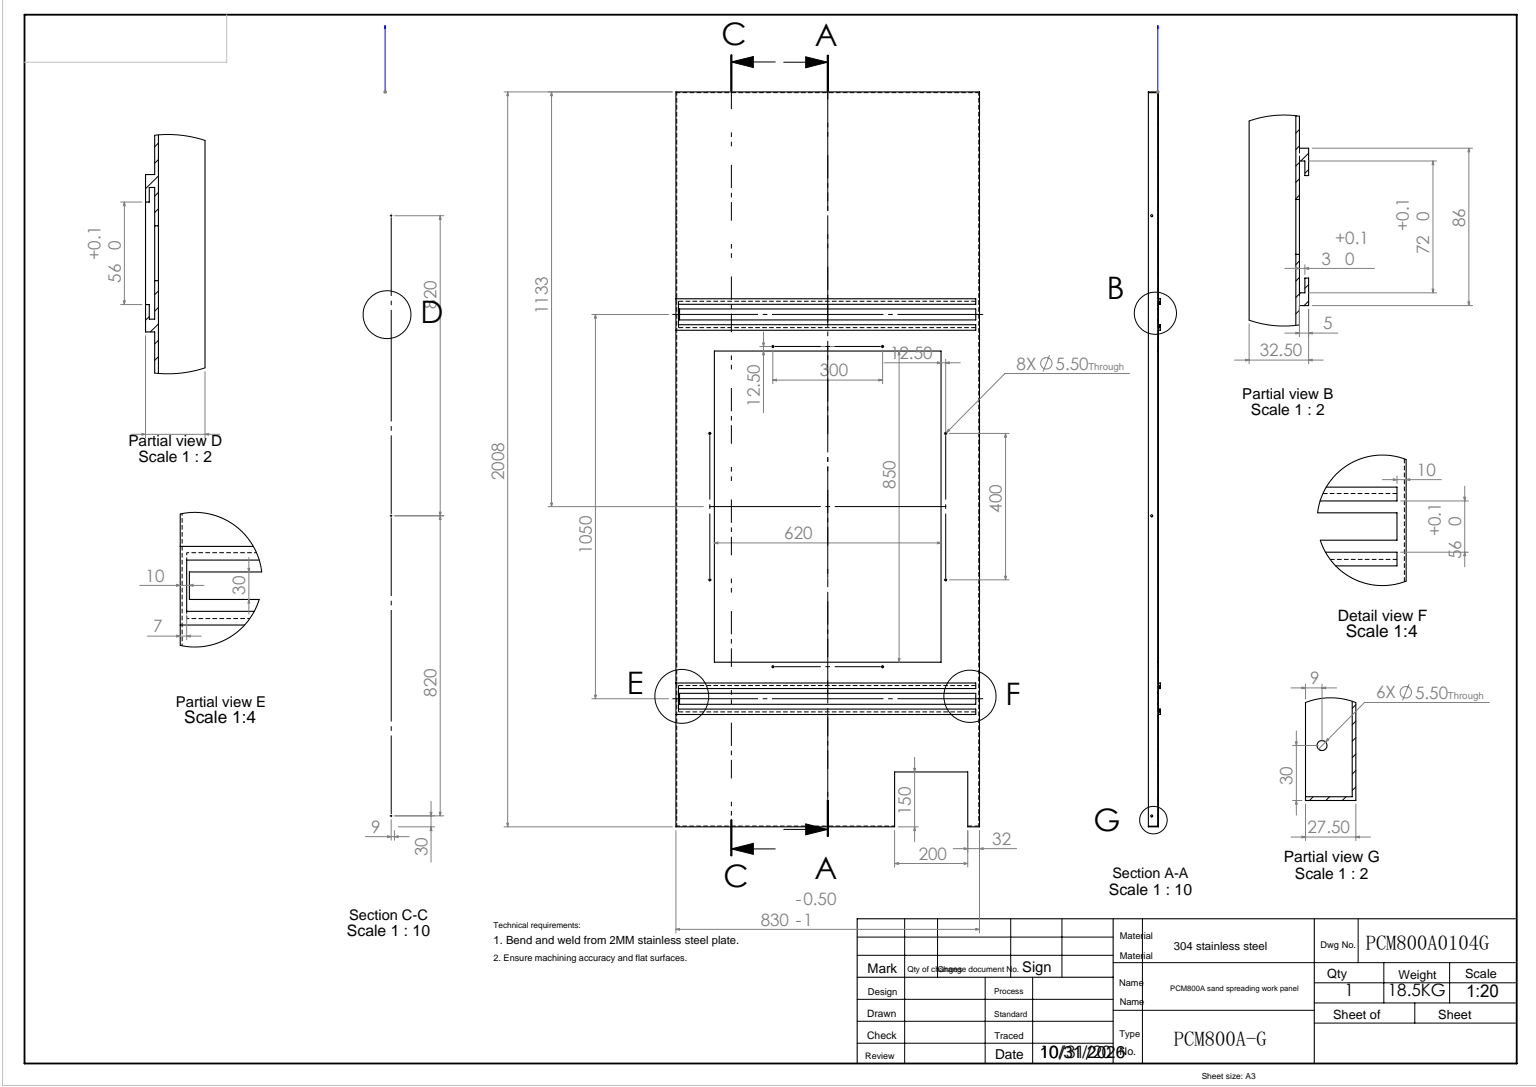
SolidWorks part; units mm, degrees
ref_plane "前视基准面" through (0, 0, 0) normal (0, 0, 1) x (1, 0, 0)
ref_plane "上视基准面" through (0, 0, 0) normal (0, 1, 0) x (1, 0, 0)
ref_plane "右视基准面" through (0, 0, 0) normal (1, 0, 0) x (0, 0, -1)
sketch "草图1" plane through (0, 0, 0) normal (0, 0, 1) x (1, 0, 0)
  line L1 (0, 0) -> (830, 0)
  line L2 (0, 0) -> (0, -2008)
  line L3 (0, -2008) -> (830, -2008)
  line L4 (830, 0) -> (830, -2008)
  line L5 (105, -708) -> (725, -708)
  line L6 (105, -708) -> (105, -1558)
  line L7 (105, -1558) -> (725, -1558)
  line L8 (725, -708) -> (725, -1558)
  dimension "D1" = 2008
  dimension "D2" = 830
  dimension "D3" = 620
  dimension "D4" = 850
  dimension "D5" = 450
  dimension "D6" = 105
extrude "凸台-拉伸1" add sketch "草图1" along normal blind 2
sketch "草图2" plane through (0, 0, 2) normal (0, 0, 1) x (1, 0, 0)
  line L1 (10, -1643) -> (820, -1643)
  line L2 (10, -1643) -> (10, -1673)
  line L3 (10, -1673) -> (820, -1673)
  line L4 (820, -1643) -> (820, -1673)
  line L5 (0, 0) -> (0, -2008) construction
  line L6 (830, -2008) -> (830, 0) construction
  line L8 (10, -593) -> (820, -593)
  line L9 (10, -593) -> (10, -623)
  line L10 (10, -623) -> (820, -623)
  line L11 (820, -593) -> (820, -623)
  line L12 (725, -708) -> (105, -708) construction
  line L13 (105, -1558) -> (725, -1558) construction
  dimension "D1" = 30
  dimension "D2" = 85
  dimension "D3" = 10
  dimension "D4" = 10
  dimension "D5" = 30
  dimension "D6" = 85
  dimension "D7" = 10
  dimension "D8" = 10
extrude "切除-拉伸1" cut sketch "草图2" against normal blind 2
sketch "草图3" plane through (0, 0, 0) normal (0, 0, 1) x (1, 0, 0)
  line L0 (830, 0) -> (0, 0) construction
  line L1 (0, -2008) -> (2, -2008)
  line L2 (0, -2008) -> (0, 0)
  line L3 (828, 0) -> (830, 0)
  line L4 (2, -2008) -> (2, 0)
  line L5 (0, -2008) -> (830, -2008) construction
  line L6 (2, 0) -> (0, 0)
  line L7 (830, 0) -> (830, -2008)
  line L8 (830, -2008) -> (828, -2008)
  line L9 (828, 0) -> (828, -2008)
  point P14 (832, -2)
  point P15 (0, -2)
  dimension "D1" = 2
  dimension "D2" = 2
extrude "凸台-拉伸2" add sketch "草图3" against normal blind 25.5
sketch "草图4" plane through (0, 0, 0) normal (0, 0, -1) x (-1, 0, 0)
  line L1 (-798, -1858) -> (-598, -1858)
  line L2 (-798, -1858) -> (-798, -2008)
  line L3 (-798, -2008) -> (-598, -2008)
  line L4 (-598, -1858) -> (-598, -2008)
  line L5 (-828, 0) -> (-828, -2008) construction
  line L6 (-2, -2008) -> (-828, -2008) construction
  dimension "D1" = 200
  dimension "D2" = 150
  dimension "D4" = 30
extrude "切除-拉伸2" cut sketch "草图4" against normal through all
sketch "草图5" plane through (0, 0, 0) normal (0, 0, -1) x (-1, 0, 0)
  line L0 (-828, 0) -> (-828, -2008) construction
  line L1 (-798, -2008) -> (-828, -2008)
  line L2 (-798, -2008) -> (-798, -2006)
  line L3 (-798, -2006) -> (-828, -2006)
  line L4 (-828, -2008) -> (-828, -2006)
  line L5 (-2, -2008) -> (-2, 0) construction
  line L6 (-598, -2008) -> (-2, -2008)
  line L7 (-598, -2008) -> (-598, -2006)
  line L8 (-598, -2006) -> (-2, -2006)
  line L9 (-2, -2008) -> (-2, -2006)
  line L11 (-828, 0) -> (-2, 0)
  line L12 (-828, 0) -> (-828, -2)
  line L13 (-828, -2) -> (-2, -2)
  line L14 (-2, 0) -> (-2, -2)
  dimension "D1" = 2
  dimension "D2" = 2
  dimension "D3" = 2
extrude "凸台-拉伸3" add sketch "草图5" along normal blind 25.5
sketch "草图7" plane through (0, 0, 2) normal (0, 0, 1) x (1, 0, 0)
  line L0 (820, -564.9973) -> (820, -580)
  line L1 (820, -564.9973) -> (0, -564.9973)
  line L2 (0, -564.9973) -> (0, -651)
  line L3 (0, -651) -> (820, -651)
  line L4 (820, -636) -> (820, -651)
  line L5 (10, -593) -> (10, -623) construction
  line L6 (7, -636) -> (820, -636)
  line L7 (820, -580) -> (7, -580)
  line L8 (10, -623) -> (820, -623) construction
  line L9 (820, -593) -> (10, -593) construction
  line L10 (7, -580) -> (7, -636)
  line L11 (820, -623) -> (820, -593) construction
  dimension "D1" = 15
  dimension "D2" = 13
  dimension "D3" = 13
  dimension "D4" = 15.0027
  dimension "D5" = 10
  dimension "D6" = 3
extrude "凸台-拉伸4" add sketch "草图7" along normal blind 5
sketch "草图8" plane through (820, 0, 0) normal (1, 0, 0) x (0, 0, -1)
  line L0 (-2, -651) -> (-2, -636) construction
  line L1 (-2, -580) -> (-5, -580)
  line L2 (-2, -580) -> (-2, -572)
  line L3 (-2, -572) -> (-5, -572)
  line L4 (-5, -580) -> (-5, -572)
  line L5 (-2, -636) -> (-5, -636)
  line L6 (-2, -636) -> (-2, -644)
  line L7 (-2, -644) -> (-5, -644)
  line L8 (-5, -636) -> (-5, -644)
  line L9 (-2, -2008) -> (-2, 0) construction
  dimension "D1" = 8
  dimension "D2" = 3
  dimension "D3" = 8
  dimension "D4" = 3
extrude "切除-拉伸3" cut sketch "草图8" against normal up to surface (813 mm away) up to face at (7, -608, 4.5)
pattern_linear "阵列(线性)1" count 2 spacing 1050 along (0, -1, 0) of "切除-拉伸3", "凸台-拉伸4"
sketch "草图9" plane through (0, 0, 0) normal (0, 0, -1) x (-1, 0, 0)
  line L10 (-737.5, -933) -> (-92.5, -933) construction
  line L11 (-737.5, -1333) -> (-92.5, -1333) construction
  line L12 (-565, -695.5) -> (-565, -1570.5) construction
  line L13 (-265, -695.5) -> (-265, -1424.9176) construction
  line L14 (-737.5, -695.5) -> (-737.5, -1570.5)
  line L15 (-737.5, -1570.5) -> (-92.5, -1570.5)
  line L16 (-92.5, -1570.5) -> (-92.5, -695.5)
  line L17 (-92.5, -695.5) -> (-737.5, -695.5)
  line L18 (-737.5, -695.5) -> (-737.5, -1570.5) construction
  line L19 (-737.5, -1570.5) -> (-92.5, -1570.5) construction
  line L20 (-92.5, -1570.5) -> (-92.5, -695.5) construction
  line L21 (-92.5, -695.5) -> (-737.5, -695.5) construction
  line L22 (-725, -1133) -> (93.2269, -1133) construction
  line L23 (-725, -1558) -> (-725, -708) construction
  line L24 (-415, -708) -> (-415, -1466.8327) construction
  line L25 (-725, -708) -> (-105, -708) construction
  circle A0 centre (-565, -695.5) radius 2.75
  circle A1 centre (-265, -695.5) radius 2.75
  circle A2 centre (-737.5, -933) radius 2.75
  circle A3 centre (-737.5, -1333) radius 2.75
  circle A4 centre (-565, -1570.5) radius 2.75
  circle A5 centre (-265, -1570.5) radius 2.75
  circle A6 centre (-92.5, -1333) radius 2.75
  circle A7 centre (-92.5, -933) radius 2.75
  dimension "D6" = 5.5
  dimension "D7" = 5.5
  dimension "D8" = 5.5
  dimension "D9" = 5.5
  dimension "D10" = 5.5
  dimension "D11" = 5.5
  dimension "D12" = 5.5
  dimension "D13" = 5.5
  dimension "D2" = 150
  dimension "D3" = 150
  dimension "D4" = 200
  dimension "D5" = 200
  dimension "D1" = 12.5
extrude "切除-拉伸4" cut sketch "草图9" against normal blind 126
sketch "草图10" plane through (0, 0, 0) normal (-1, 0, 0) x (0, 0, 1)
  line L0 (-16.5, -1848) -> (-16.5, 282.4928) construction
  line L2 (2, -2008) -> (-25.5, -2008) construction
  line L4 (-25.5, 0) -> (-25.5, -2008) construction
  circle A0 centre (-16.5, -1978) radius 2.75
  circle A1 centre (-16.5, -1158) radius 2.75
  circle A2 centre (-16.5, -338) radius 2.75
  dimension "D1" = 5.5
  dimension "D2" = 30
  dimension "D4" = 5.5
  dimension "D5" = 5.5
  dimension "D6" = 820
  dimension "D7" = 820
  dimension "D3" = 9
extrude "切除-拉伸5" cut sketch "草图10" against normal blind 1163
